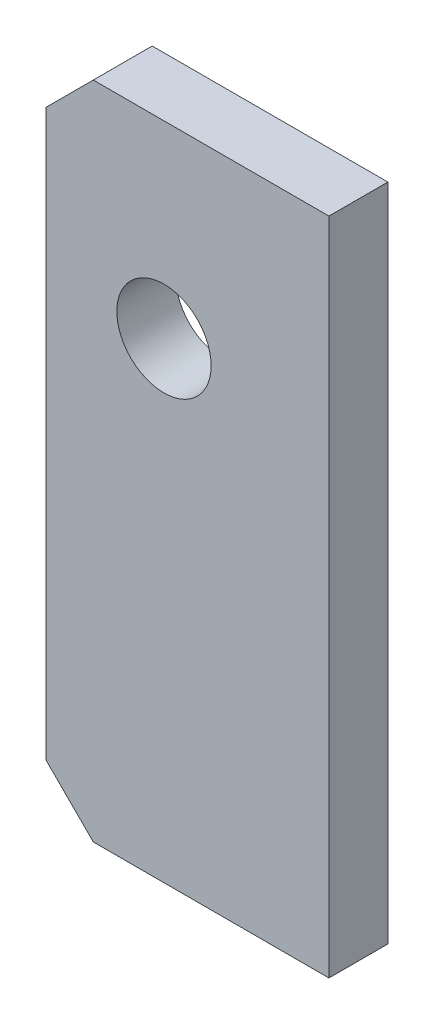
SolidWorks part; units mm, degrees
ref_plane "前视基准面" through (0, 0, 0) normal (0, 0, 1) x (1, 0, 0)
ref_plane "上视基准面" through (0, 0, 0) normal (0, 1, 0) x (1, 0, 0)
ref_plane "右视基准面" through (0, 0, 0) normal (1, 0, 0) x (0, 0, -1)
sketch "草图1" plane through (0, 0, 0) normal (0, 0, 1) x (1, 0, 0)
  line L1 (0, 0) -> (-120, 0)
  line L2 (0, 0) -> (0, 280)
  line L3 (0, 280) -> (-120, 280)
  line L4 (-120, 0) -> (-120, 280)
  dimension "D1" = 120
  dimension "D2" = 280
extrude "凸台-拉伸1" add sketch "草图1" along normal blind 25
sketch "草图2" plane through (0, 0, 25) normal (0, 0, 1) x (1, 0, 0)
  line L0 (-120, 280) -> (-120, 0) construction
  line L1 (0, 280) -> (-120, 280) construction
  circle A0 centre (-70, 200) radius 20
  dimension "D3" = 40
  dimension "D1" = 50
  dimension "D2" = 80
extrude "切除-拉伸1" cut sketch "草图2" against normal through all both and the other way through all
chamfer "倒角1" distance 20 angle 45 2 edges at (-120, 0, 12.5) (-120, 280, 12.5)
